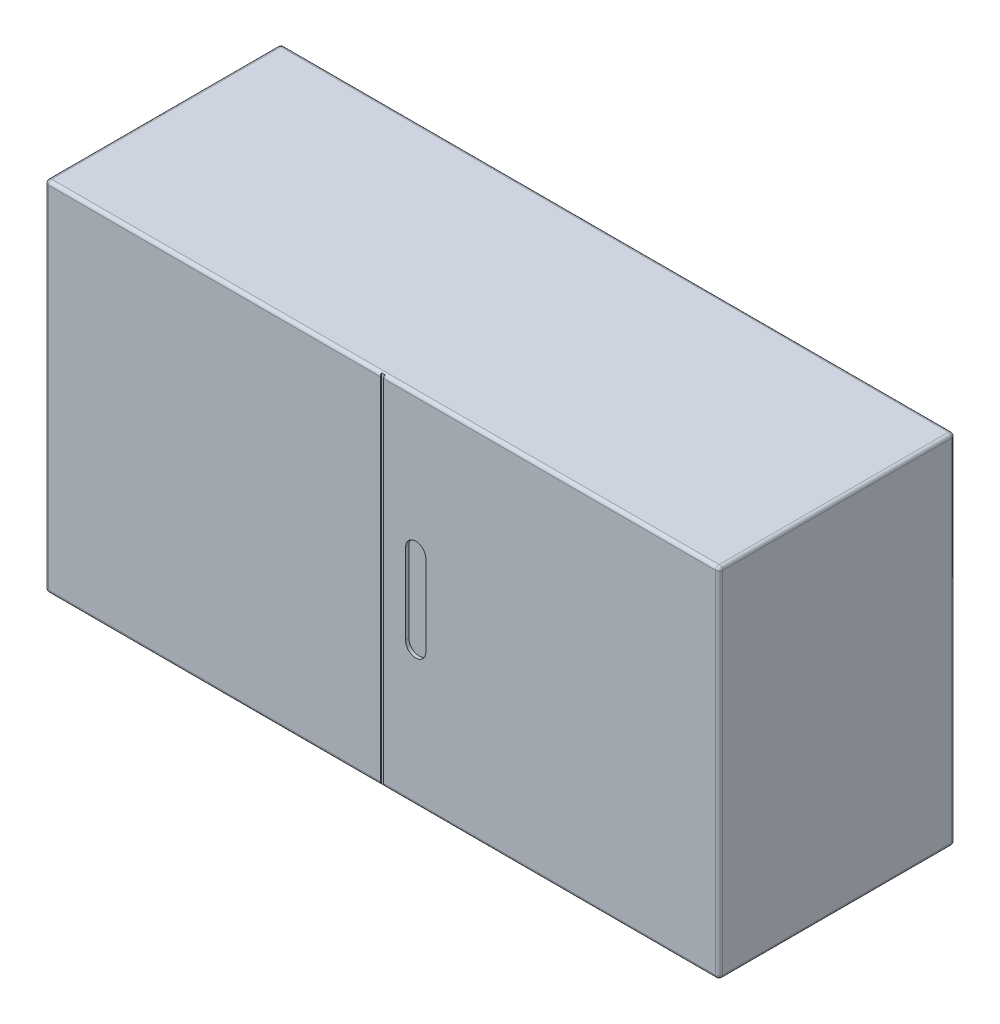
SolidWorks part; units mm, degrees
ref_plane "Front Plane" through (0, 0, 0) normal (0, 0, 1) x (1, 0, 0)
ref_plane "Top Plane" through (0, 0, 0) normal (0, 1, 0) x (1, 0, 0)
ref_plane "Right Plane" through (0, 0, 0) normal (1, 0, 0) x (0, 0, -1)
sketch "Sketch1" plane through (0, 0, 0) normal (0, 0, 1) x (1, 0, 0)
  line L1 (-500, -265) -> (500, -265)
  line L2 (-500, -265) -> (-500, 265)
  line L3 (-500, 265) -> (500, 265)
  line L4 (500, -265) -> (500, 265)
  line L5 (-500, -265) -> (500, 265) construction
  line L6 (-500, 265) -> (500, -265) construction
  point P0 (0, 0)
  dimension "D1" = 530
  dimension "D2" = 1000
extrude "Boss-Extrude1" add sketch "Sketch1" along normal blind 350
fillet "Fillet1" radius 5 12 edges at (0, 265, 0) (-500, 0, 0) (0, -265, 0) (500, 0, 0) (0, -265, 350) (-500, 0, 350) (0, 265, 350) (500, 0, 350) (-500, 265, 175) (500, 265, 175) (-500, -265, 175) (500, -265, 175)
sketch "Sketch3" plane through (0, 0, 350) normal (0, 0, 1) x (1, 0, 0)
  line L0 (0, 265) -> (0, -265) construction
  line L1 (-495, 265) -> (495, 265) construction
  line L2 (495, -265) -> (-495, -265) construction
  line L4 (-2.5, -265) -> (2.5, -265)
  line L5 (-2.5, -265) -> (-2.5, 265)
  line L6 (-2.5, 265) -> (2.5, 265)
  line L7 (2.5, -265) -> (2.5, 265)
  line L8 (-2.5, -265) -> (2.5, 265) construction
  line L9 (-2.5, 265) -> (2.5, -265) construction
  point P6 (0, 0)
  dimension "D1" = 5
extrude "Cut-Extrude2" cut sketch "Sketch3" against normal blind 2
sketch "Sketch4" plane through (0, 0, 350) normal (0, 0, 1) x (1, 0, 0)
  line L0 (50, 60) -> (50, -60) construction
  line L1 (65, 60) -> (65, -60)
  line L2 (35, 60) -> (35, -60)
  arc A0 (65, 60) -> (35, 60) centre (50, 60) ccw
  arc A1 (35, -60) -> (65, -60) centre (50, -60) ccw
  point P2 (50, 0)
  dimension "D1" = 30
  dimension "D2" = 120
  dimension "D3" = 50
extrude "Cut-Extrude3" cut sketch "Sketch4" against normal blind 5
sketch "Sketch5" plane through (0, -265, 0) normal (0, -1, 0) x (1, 0, 0)
  line L0 (-500, 175) -> (500, 175) construction
  line L1 (-500, 5) -> (-500, 345) construction
  line L2 (500, 345) -> (500, 5) construction
  line L4 (-225, 145) -> (225, 145)
  line L5 (-225, 145) -> (-225, 205)
  line L6 (-225, 205) -> (225, 205)
  line L7 (225, 145) -> (225, 205)
  line L8 (-225, 145) -> (225, 205) construction
  line L9 (-225, 205) -> (225, 145) construction
  point P6 (0, 175)
  dimension "D1" = 450
  dimension "D2" = 60
extrude "Cut-Extrude4" cut sketch "Sketch5" against normal blind 1
fillet "Fillet2" radius 10 4 edges at (-225, -264.5, 205) (-225, -264.5, 145) (225, -264.5, 205) (225, -264.5, 145)
sketch "Sketch6" plane through (0, -265, 0) normal (0, -1, 0) x (1, 0, 0)
  circle A0 centre (-730, 350) radius 730
  circle A1 centre (730, 350) radius 730
  line M9 (495, 345) -> (-495, 345)
  line M11 (-495, 5) -> (495, 5)
  line M12 (495, 5) -> (495, 345)
extrude "Boss-Extrude2" [suppressed] add sketch "Sketch6" against normal up to surface (530 mm away) contours A1 M9 M12 M11
